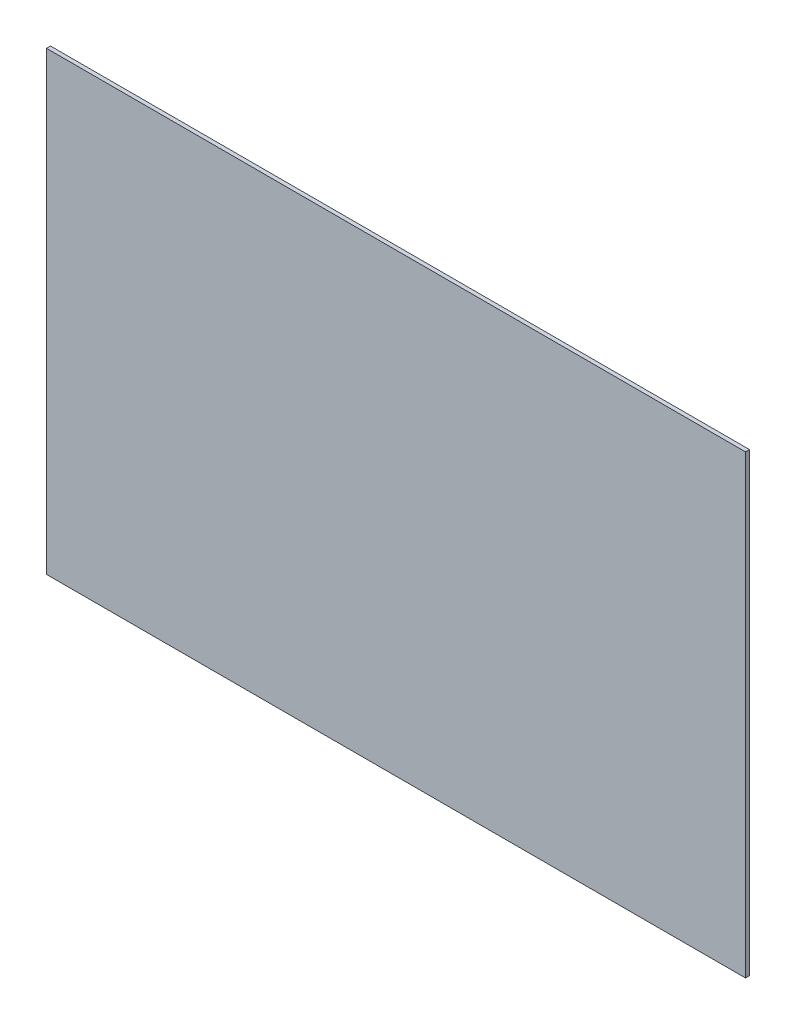
from build123d import *

# Parameters (mm, degrees)
SKETCH_1_W      = 876
SKETCH_1_H      = 571
EXTRUDE_1_DEPTH = 5


with BuildPart() as part:
    # 草图1 → 凸台-拉伸1 (new body)
    with BuildSketch(Plane.XY):
        Rectangle(SKETCH_1_W, SKETCH_1_H)
    extrude(amount=EXTRUDE_1_DEPTH)


solid = part.part
